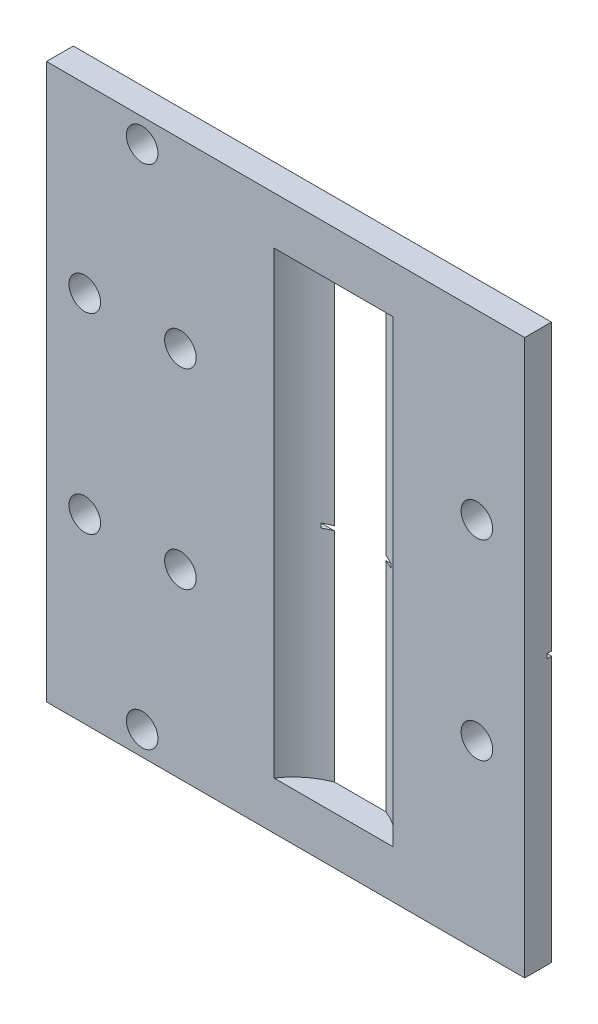
SolidWorks part; units mm, degrees
ref_plane "前视基准面" through (0, 0, 0) normal (0, 0, 1) x (1, 0, 0)
ref_plane "上视基准面" through (0, 0, 0) normal (0, 1, 0) x (1, 0, 0)
ref_plane "右视基准面" through (0, 0, 0) normal (1, 0, 0) x (0, 0, -1)
sketch "草图1" plane through (0, 0, 0) normal (0, 0, 1) x (1, 0, 0)
  line L1 (-39.0078, 21.4373) -> (10.9922, 21.4373)
  line L2 (-39.0078, 21.4373) -> (-39.0078, -36.5627)
  line L3 (-39.0078, -36.5627) -> (10.9922, -36.5627)
  line L4 (10.9922, 21.4373) -> (10.9922, -36.5627)
  dimension "D1" = 58
  dimension "D2" = 50
extrude "凸台-拉伸1" add sketch "草图1" along normal blind 2.8
sketch "草图2" plane through (0, 0, 2.8) normal (0, 0, 1) x (1, 0, 0)
  line L0 (10.9922, 21.4373) -> (-39.0078, 21.4373) construction
  line L1 (-39.0078, 21.4373) -> (-39.0078, -36.5627) construction
  line L2 (10.9922, -36.5627) -> (10.9922, 21.4373) construction
  line L3 (-39.0078, -36.5627) -> (10.9922, -36.5627) construction
  circle A0 centre (-29.0078, 18.9373) radius 1.65
  circle A1 centre (-35.0078, 2.4373) radius 1.65
  circle A2 centre (-25.0078, 2.4373) radius 1.65
  circle A3 centre (5.9922, 2.4373) radius 1.65
  circle A4 centre (-35.0078, -17.5627) radius 1.65
  circle A5 centre (-25.0078, -17.5627) radius 1.65
  circle A6 centre (-29.0078, -34.0627) radius 1.65
  circle A7 centre (5.9922, -17.5627) radius 1.65
  dimension "D9" = 3.3
  dimension "D10" = 3.3
  dimension "D11" = 3.3
  dimension "D12" = 3.3
  dimension "D13" = 3.3
  dimension "D14" = 3.3
  dimension "D15" = 3.3
  dimension "D16" = 3.3
  dimension "D1" = 19
  dimension "D2" = 4
  dimension "D3" = 2.5
  dimension "D4" = 10
  dimension "D5" = 19
  dimension "D6" = 14
  dimension "D7" = 5
  dimension "D8" = 19
  dimension "D17" = 19
  dimension "D18" = 19
  dimension "D19" = 19
  dimension "D20" = 4
  dimension "D21" = 10
  dimension "D22" = 14
  dimension "D23" = 2.5
  dimension "D24" = 5
extrude "切除-拉伸1" cut sketch "草图2" against normal through all
sketch "草图3" plane through (10.9922, 0, 0) normal (1, 0, 0) x (0, 0, -1)
  line L0 (0, -36.5627) -> (0, 21.4373) construction
  line L1 (0, -8.8127) -> (-0.45, -8.8127)
  line L2 (0, -8.8127) -> (0, -8.3627)
  line L3 (0, -8.3627) -> (-0.45, -8.3627)
  line L4 (-0.45, -8.8127) -> (-0.45, -8.3627)
  dimension "D1" = 0.45
  dimension "D2" = 0.45
  dimension "D3" = 29.8
extrude "切除-拉伸2" cut sketch "草图3" against normal through all
ref_plane "基准面4" through (0, 16.4373, 0) normal (0, 1, 0) x (1, 0, 0)
sketch "草图5" plane through (0, 16.4373, 0) normal (0, 1, 0) x (1, 0, 0)
  line L0 (10.9922, -2.8) -> (-39.0078, -2.8) construction
  line L1 (10.9922, -2.8) -> (10.9922, 0) construction
  line L2 (-2.7941, -2.8) -> (-15.2215, -2.8)
  line L3 (-11.7004, 0) -> (-6.4082, 0.0351)
  line L4 (10.9922, 0) -> (-39.0078, 0) construction
  arc A0 (-2.7941, -2.8) -> (-6.4082, 0.0351) centre (-9.0078, -7) ccw
  arc A1 (-11.7004, 0) -> (-15.2215, -2.8) centre (-9.0078, -7) ccw
  dimension "D3" = 15
  dimension "D1" = 4.2
  dimension "D2" = 20
extrude "切除-拉伸3" cut sketch "草图5" against normal blind 48
